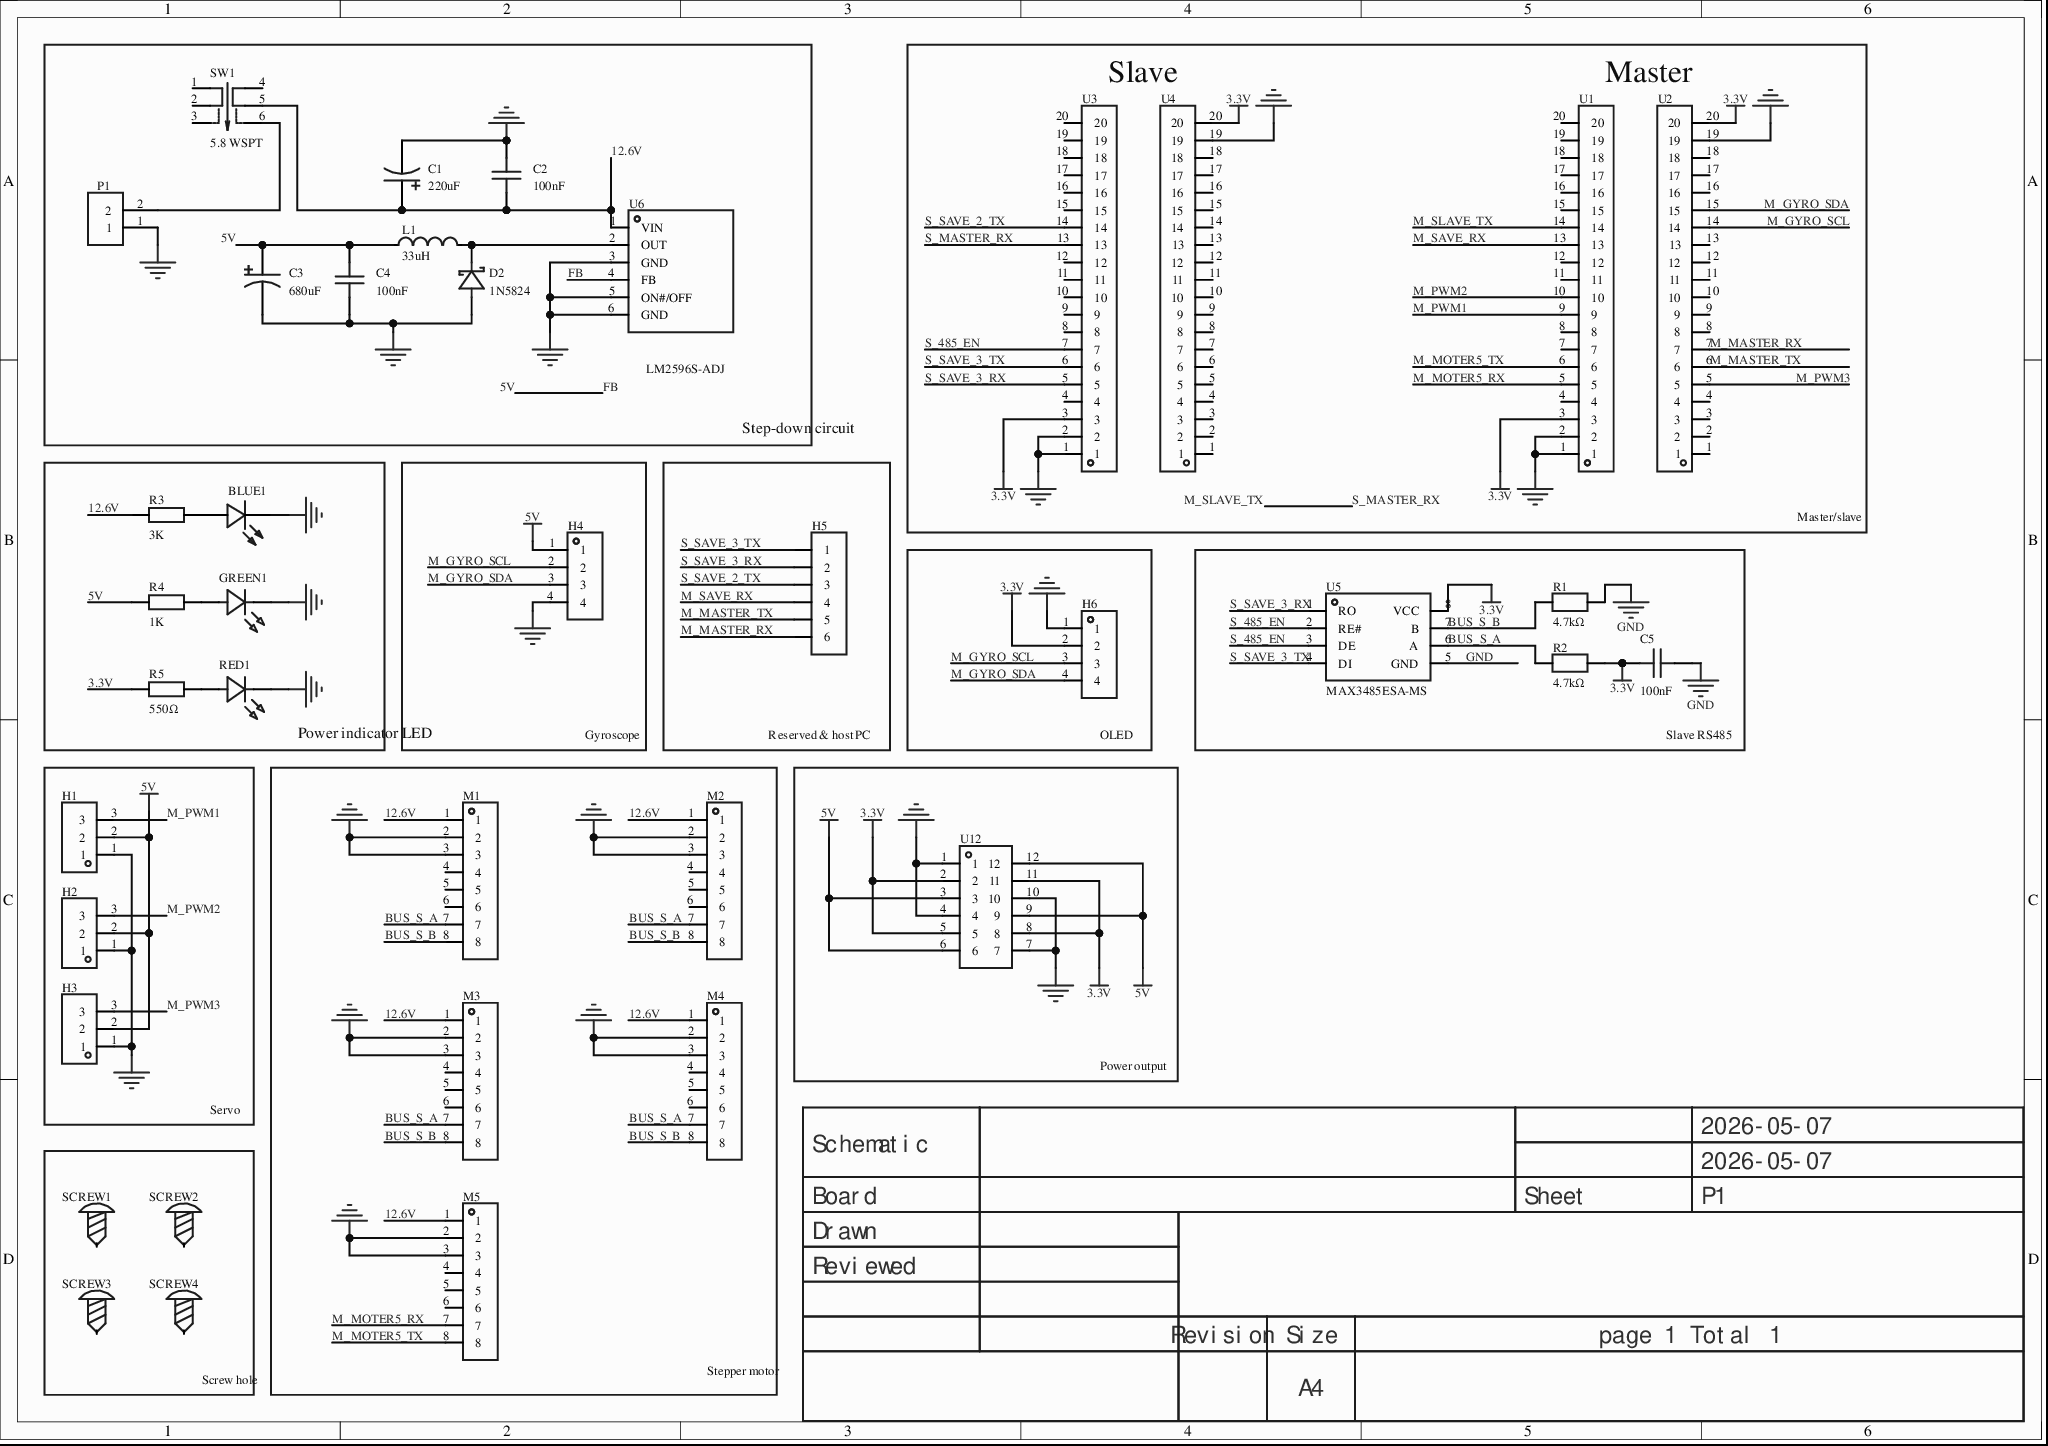
[diagram p0: MISC50151-3.schdoc]
# Altium project MISC50151-2.PrjPcb
1 sheet, 39 parts. Net scope: global (net labels, ports and power ports of the same name join across sheets).
Board file: MISC50151.pcbdoc

## Sheet MISC50151-3.schdoc
size 297 x 209 mm; Version: V1.0; @Project Name: MISC50151; @Page Count: 1; @Update Date: 2026-05-07; @Create Date: 2026-05-07; @Schematic Name: MISC50151; @Page No: 1; @Create Time: 22:11:46; @Update Time: 23:26:42; @Board Name: MISC50151

### Parts
BLUE1  SZYY0603B  [LED0603-R-RD_BLUE]  (value not drawn)
C1  220uF  [CAP-SMD_BD10.0-L10.3-W10.3-FD]
C2  100nF  [C0805]
C3  680uF  [CAP-SMD_BD8.0-L8.3-W8.3-FD]
C4  100nF  [C0805]
C5  100nF  [C0603]
D2  1N5824  [DO-27_BD5.3-L8.4-P12.40-D1.3-RD]
GREEN1  XL-1608PGC-06  [LED0603-RD_GREEN]  (value not drawn)
H1  PZ254V-11-03P  [HDR-TH_3P-P2.54-V-M]  (value not drawn)
H2  PZ254V-11-03P  [HDR-TH_3P-P2.54-V-M]  (value not drawn)
H3  PZ254V-11-03P  [HDR-TH_3P-P2.54-V-M]  (value not drawn)
H4  PZ254V-11-04P  [HDR-TH_4P-P2.54-V-M]  (value not drawn)
H5  2.54-1x6P straight pin  [HDR-TH_6P-P2.54-V-M-1]  (value not drawn)
H6  PZ254V-11-04P  [HDR-TH_4P-P2.54-V-M]  (value not drawn)
L1  33uH  [IND-SMD_L13.45-W12.6]
M1  ZX-XH2.54-8PWZ  [CONN-TH_8P-P2.50_ZX-XH2.54-8PWZ]  (value not drawn)
M2  ZX-XH2.54-8PWZ  [CONN-TH_8P-P2.50_ZX-XH2.54-8PWZ]  (value not drawn)
M3  ZX-XH2.54-8PWZ  [CONN-TH_8P-P2.50_ZX-XH2.54-8PWZ]  (value not drawn)
M4  ZX-XH2.54-8PWZ  [CONN-TH_8P-P2.50_ZX-XH2.54-8PWZ]  (value not drawn)
M5  ZX-XH2.54-8PWZ  [CONN-TH_8P-P2.50_ZX-XH2.54-8PWZ]  (value not drawn)
P1  WJ500V-5.08-2P  [CONN-TH_2P-P5.00_WJ500V-5.08-2P]  (value not drawn)
R1  4.7kΩ  [R0805]
R2  4.7kΩ  [R0805]
R3  3K  [R0805]
R4  1K  [R0805]
R5  550Ω  [R0805]
RED1  XL-1608SURC-06  [LED0603-RD_RED]  (value not drawn)
SCREW1  (no value)  [M3螺丝]
SCREW2  (no value)  [M3螺丝]
SCREW3  (no value)  [M3螺丝]
SCREW4  (no value)  [M3螺丝]
SW1  5.8 WSPT  [SW-TH_6P-L5.8-W5.8-P2.00-LS4.5-TL_K8-5851E-L1]
U1  ZX-PM2.54-1-20PY  [HDR-TH_20P-P2.54-V-F]  (value not drawn)
U2  ZX-PM2.54-1-20PY  [HDR-TH_20P-P2.54-V-F]  (value not drawn)
U3  ZX-PM2.54-1-20PY  [HDR-TH_20P-P2.54-V-F]  (value not drawn)
U4  ZX-PM2.54-1-20PY  [HDR-TH_20P-P2.54-V-F]  (value not drawn)
U5  MAX3485ESA-MS  [SO-8_L4.9-W3.9-P1.27-LS5.9-BL]
U6  LM2596S-ADJ  [TO-263-5_L10.2-W8.6-P1.70-LS14.4-BR]
U12  HX PZ2.54-3x4P ZZ  [HDR-TH_12P-P2.54-V-M-R3-C4-S2.54]  (value not drawn)

### Blocks framed on the sheet
Step-down circuit: C1-C4 D2 L1 P1 SW1 U6
Power indicator LED: BLUE1 GREEN1 R3-R5 RED1
Gyroscope: H4
Reserved & host PC: H5
OLED: H6
Slave RS485: C5 R1 R2 U5
Servo: H1-H3
Stepper motor: M1-M5
Power output: U12
Screw hole: SCREW1-SCREW4

### Nets
3.3V: C5.1 H6.2 R2.2 R5.2 U1.3 U2.20 U3.3 U4.20 U5.8(VCC) U12.2 U12.5 U12.8 U12.11
5V: C3.1 C4.2 H1.2 H2.2 H3.2 H4.1 L1.1 R4.2 U6.4(FB) U12.3 U12.6 U12.9 U12.12  [also labelled FB]
GND: BLUE1.2(-) C1.2 C2.1 C3.2 C4.1 C5.2 D2.2(A) GREEN1.1(K) H1.1 H2.1 H3.1 H4.4 H6.1 M1.2 M1.3 M2.2 M2.3 M3.2 M3.3 M4.2 M4.3 M5.2 M5.3 P1.1 R1.2 RED1.1(K) U1.1 U1.2 U2.19 U3.1 U3.2 U4.19 U5.5(GND) U6.3(GND) U6.5(ON#/OFF) U6.6(GND) U12.1 U12.4 U12.7 U12.10
12.6V: C1.1 C2.2 M1.1 M2.1 M3.1 M4.1 M5.1 R3.2 SW1.5 U6.1(VIN)
BUS_S_A: M1.7 M2.7 M3.7 M4.7 R2.1 U5.6(A)
BUS_S_B: M1.8 M2.8 M3.8 M4.8 R1.1 U5.7(B)
M_GYRO_SCL: H4.2 H6.3 U2.14
M_GYRO_SDA: H4.3 H6.4 U2.15
M_MASTER_RX: H5.6 U2.7
M_MASTER_TX: H5.5 U2.6
M_MOTER5_RX: M5.7 U1.5
M_MOTER5_TX: M5.8 U1.6
M_PWM1: H1.3 U1.9
M_PWM2: H2.3 U1.10
M_PWM3: H3.3 U2.5
M_SAVE_RX: H5.4 U1.13
M_SLAVE_TX: U1.14 U3.13  [also labelled S_MASTER_RX]
S_485_EN: U3.7 U5.2(RE#) U5.3(DE)
S_SAVE_2_TX: H5.3 U3.14
S_SAVE_3_RX: H5.2 U3.5 U5.1(RO)
S_SAVE_3_TX: H5.1 U3.6 U5.4(DI)
NetBLUE1_1: BLUE1.1(+) R3.1
NetD2_1: D2.1(K) L1.2 U6.2(OUT)
NetGREEN1_2: GREEN1.2(A) R4.1
NetP1_2: P1.2 SW1.6
NetR5_1: R5.1 RED1.2(A)

Not connected (* = marked no-connect by the designer): M1 4* 5* 6*; M2 4* 5* 6*; M3 4* 5* 6*; M4 4* 5* 6*; M5 4* 5* 6*; SCREW1 1*; SCREW2 1*; SCREW3 1*; SCREW4 1*; SW1 1* 2* 3* 4*; U1 4* 7* 8* 11* 12* 15* 16* 17* 18* 19* 20*; U2 1* 2* 3* 4* 8* 9* 10* 11* 12* 13* 16* 17* 18*; U3 4* 8* 9* 10* 11* 12* 15* 16* 17* 18* 19* 20*; U4 1* 2* 3* 4* 5* 6* 7* 8* 9* 10* 11* 12* 13* 14* 15* 16* 17* 18*

### Notes on the sheet
- Slave
- Master
- Master/slave
- 2026-05-07
- Schematic
- Board
- Sheet
- P1
- Drawn
- Reviewed
- Revision
- Size
- A4
- page 1 Total 1

### Library data of the parts
BLUE1 = SZYY0603B: Emitted color: Blue; Power: 100mW; Forward current: 5mA; Dominant wavelength: 460nm~475nm; Diode configuration: -; Lens color: Colorless transparent lens; Color temperature: -; Viewing angle: 120°; Packaging: -; Operating temperature: -40℃~+85℃;; Manufacturer: yongyu(永裕光电); AddInBom: yes; ModelId: 084ad08e1cd342ca871cc791b88f1a3a; ModelTransform: 63.7794,31.496,0,0,0,0,0,0,0; Peak Wavelength: 469nm; Symbol: SZYY0603B; Device: SZYY0603B; LCSC Part Name: 蓝灯; SupplierPart: C434421; ManufacturerPart: SZYY0603B; Supplier Footprint: 0603; JLCPCB Part Class: Extended library; Datasheet: https://example.com/upload/public/pdf/source/20191204/C434421_A4F05E4DF64B0F36639806529E783B5C.pdf; Supplier: LCSC; ConvertToPcb: yes; FootprintName: LED0603-R-RD_BLUE; ModelName: LED0603-R-RD_BLUE; Emitted Color: Blue; Power Dissipation: 100mW; Forward Current: 5mA; Dominant Wavelength: 460nm~475nm; Diode Configuration: -; Lens Color: Colorless transparent lens; Color Temperature: -; Viewing Angle: 120°; Mounting Sytle: -; Operating Temperature: -40℃~+85℃
C1 = EEEFK1H221P: Capacitance: 220uF; Tolerance: ±20%; Rated voltage: 50V; Capacitor body diameter: 10mm; Capacitor body length: 10.2mm; Ripple current: -; Equivalent series resistance: -; Operating life: 2000hrs@105℃; Operating temperature: -45℃~+105℃;; Manufacturer: PANASONIC(松下); AddInBom: yes; ModelId: b23815befd5e4172abc55cc8ac2654de; ModelTransform: 456.692,405.511,0,180,0,0,0,0,0; Device: EEEFK1H221P; Symbol: EEEFK1H221P; LCSC Part Name: 220uF±20%50V; SupplierPart: C178549; ManufacturerPart: EEEFK1H221P; Supplier Footprint: SMD,10x10.2mm; JLCPCB Part Class: ExtendedPart; Datasheet: https://example.com/upload/public/pdf/source/20180329/C178549_6E0EC09DB3BC10F05F8D4E4FCB841907.pdf; Supplier: LCSC; ConvertToPcb: yes; FootprintName: CAP-SMD_BD10.0-L10.3-W10.3-FD; ModelName: CAP-SMD_BD10.0-L10.3-W10.3-FD; Value: 220uF; Rated Voltage: 50V; φD: 10mm; L: 10.2mm; Ripple Current: -; Equivalent Series Resistance(ESR): -; Lifetime @ Temp: 2000hrs@105℃; Operating Temperature: -45℃~+105℃
C2 C4 = CAP_0805: ConvertToPcb: yes; SymbolName: CapAcitance; ModelId: 1ba041120af144c991958decab20d241; ModelName: C0805_L2.0-W1.3-H1.3; ModelTransform: 78.74,51.181,0,0,0,0,0,0.0005,0; Device: CAP_0805; AddInBom: yes; Supplier Footprint: 0805; FootprintName: C0805; Value: 100nF
C3 = EEEFP1V221AP: Capacitance: 220uF; Tolerance: ±20%; Rated voltage: 35V; Capacitor body diameter: 8mm; Capacitor body length: 10.2mm; Ripple current: -; Equivalent series resistance: -; Operating life: 2000hrs@105℃; Operating temperature: -45℃~+105℃;; Manufacturer: PANASONIC(松下); AddInBom: yes; ModelId: 5c9301d64f8b45ea89e061ac72e6cbf7; ModelTransform: 393.7,326.771,0,180,0,0,0,0,0; Value: 680uF; Device: EEEFP1V221AP; Symbol: EEEFP1V221AP; LCSC Part Name: 220uF ±20% 35V; ManufacturerPart: EEEFP1V221AP; Supplier Footprint: SMD,8x10.2mm; JLCPCB Part Class: Extended Part; Datasheet: https://example.com/upload/public/pdf/source/20181130/C278406_CB9CD87BC4579E70B6A89BF3334E5E7E.pdf; Supplier: LCSC; ConvertToPcb: yes; FootprintName: CAP-SMD_BD8.0-L8.3-W8.3-FD; ModelName: CAP-SMD_BD8.0-L8.3-W8.3-FD; Rated Voltage: 35V; φD: 8mm; L: 10.2mm; Ripple Current: -; Equivalent Series Resistance(ESR): -; Lifetime @ Temp: 2000hrs@105℃; Operating Temperature: -45℃~+105℃
C5 = CGA0603X7R104K500JT: Capacitance: 100nF; Tolerance: ±10%; Rated voltage: 50V; Temperature coefficient: X7R;; Manufacturer: HRE(芯声); AddInBom: yes; ModelId: ac125912035d415993ca9572d50418b10819f05c4eef4c71ace90d822a990e87; ModelName: C0603_L1.6-W0.8-H0.8; ModelTransform: 62.992,31.496,0,0,0,0,0,0,0; Symbol: CGA0603X7R104K500JT; Device: CGA0603X7R104K500JT; LCSC Part Name: 100nF ±10% 50V; SupplierPart: C6119867; ManufacturerPart: CGA0603X7R104K500JT; Supplier Footprint: 0603; JLCPCB Part Class: Extended Part; Datasheet: https://example.com/datasheet/CGA0603X7R104K500JT/7062573.html; Supplier: LCSC; ConvertToPcb: yes; FootprintName: C0603; Value: 100nF; Voltage Rating: 50V; Temperature Coefficient: X7R
D2 = 1N5824_C7503125: Diode configuration: Single; Forward voltage drop (Vf): 550mV@5A; DC reverse voltage (Vr): 30V; Rectified current: 5A;; Manufacturer: FUXINSEMI(富芯森美); AddInBom: yes; ModelId: 34c822afc58c4389bef282cc7fc2257f; ModelTransform: 578.739,207.771,0,0,0,0,0,0,-196.85; Reverse Leakage Current (Ir): 500uA@30V; Operating Junction Temperature Range: -55℃~+150℃; Non-Repetitive Peak Forward Surge Current: 150A; Symbol: 1N5824_C7503125; Device: 1N5824_C7503125; LCSC Part Name: 电压:30V 电流:5A; SupplierPart: C7503125; ManufacturerPart: 1N5824; Supplier Footprint: DO-201AD; JLCPCB Part Class: Extended library; Datasheet: https://example.com/datasheet/1N5824/8591231.html; Supplier: LCSC; ConvertToPcb: yes; FootprintName: DO-27_BD5.3-L8.4-P12.40-D1.3-RD; ModelName: DO-27_BD5.3-L8.4-P12.40-D1.3-RD; Diode Configuration: Single; Voltage - Forward(Vf@If): 550mV@5A; Voltage - DC Reverse(Vr): 30V; Current - Rectified: 5A
GREEN1 = XL-1608PGC-06: Lamp head type: -; Emitted color: Emerald green; Forward voltage (Vf): 2.6V~3V; Power: -; Forward current: -; Wavelength: 515nm~530nm; Diode configuration: -; Lens color: Green lens; Color temperature: -; Luminous intensity: 900mcd; Viewing angle: 120°; Packaging: SMD; Operating temperature: -;; Manufacturer: XINGLIGHT(成兴光); AddInBom: yes; ModelId: 7761174b67d9475ab0dbce38062fb2f9; ModelTransform: 63.7794,31.496,0,0,0,0,0,0,0; Peak Wavelength: 525nm; Symbol: XL-1608PGC-06; Device: XL-1608PGC-06; LCSC Part Name: 0603加粉翠绿0.6T贴片式发光二极管; SupplierPart: C7371905; ManufacturerPart: XL-1608PGC-06; Supplier Footprint: 0603; JLCPCB Part Class: Extended library; Datasheet: https://example.com/datasheet/XL-1608PGC-06/8342977.html; Supplier: LCSC; ConvertToPcb: yes; FootprintName: LED0603-RD_GREEN; ModelName: LED0603-RD_GREEN; Lamp Holder Type: -; Illumination Color: Emerald green; Voltage - Forward(Vf): 2.6V~3V; Power(Watts): -; Forward Current: -; Wavelength - Dominant: 515nm~530nm; Diode Configuration: -; Lens Color: Green lens; Color Temperature: -; Luminous Intensity: 900mcd; Viewing Angle: 120°; Mounting Style: SMD; Operating Temperature: -
H1-H3 = PZ254V-11-03P: Pin structure: 1x3P; Pitch: 2.54mm; Row spacing: -; Round/square pin: Square pin; Mounting style: Through-hole; Rows: Single row; Total pins: 3P; Rated current: 3A; Rated voltage: 250V; Mating pin length: 6mm; Plastic height: 2.5mm; Tail length: 3mm; Operating temperature: -40℃~+105℃; Color: Black;; Manufacturer: XFCN(兴飞); Symbol: PZ254V-11-03P_C2937625; AddInBom: yes; ModelId: bb473b6d38ff42a99216a4fcdbdcc4cb; ModelName: HDR-TH_3P-P2.54-M-LI-1X3P; ModelTransform: 299.9994,100,0,0,0,0,0,0,-118.11; Device: PZ254V-11-03P; LCSC Part Name: 1x3P 间距:2.54mm 方针 直插; SupplierPart: C2937625; ManufacturerPart: PZ254V-11-03P; Supplier Footprint: 插件,P=2.54mm; JLCPCB Part Class: Extended library; Datasheet: https://example.com/datasheet/PZ254V-11-03P/3293280.html; Supplier: LCSC; ConvertToPcb: yes; FootprintName: HDR-TH_3P-P2.54-V-M; Pin Structure: 1x3P; Row Spacing: -; Circluar Pins/Square Pins: Square pin; Mounting Type: Through-hole; Number of Rows: Single row; Number of Pins: 3P; Current Rating: 3A; Voltage Rating (Max): 250V; Length of Mating Pin: 6mm; Insulation Height: 2.5mm; Length of End Connection Pin: 3mm; Operating Temperature: -40℃~+105℃; Color: Black
H4 H6 = PZ254V-11-04P: Pin structure: 1x4P; Pitch: 2.54mm; Row spacing: -; Round/square pin: Square pin; Mounting style: Through-hole; Rows: Single row; Total pins: 4P; Rated current: 3A; Rated voltage: 250V; Mating pin length: 6mm; Plastic height: 2.5mm; Tail length: 3mm; Contact material: -; Operating temperature: -40℃~+105℃;; Manufacturer: XFCN(兴飞); Symbol: PZ254V-11-04P_C2691448; AddInBom: yes; ModelId: 112f4d05e8d64e99ab9a333894bea4f9; ModelName: HDR-TH_4P-P2.54-M-LI-1X4P; ModelTransform: 399.999,104.7242,0,0,0,0,0,0,-118.11; Device: PZ254V-11-04P; LCSC Part Name: 1x4P 间距:2.54mm 方针 直插; SupplierPart: C2691448; ManufacturerPart: PZ254V-11-04P; Supplier Footprint: 插件,P=2.54mm; JLCPCB Part Class: Extended library; Datasheet: https://example.com/datasheet/PZ254V-11-04P/2801085.html; Supplier: LCSC; ConvertToPcb: yes; FootprintName: HDR-TH_4P-P2.54-V-M; Pin Structure: 1x4P; Row Spacing: -; Circluar Pins/Square Pins: Square pin; Mounting Type: Through-hole; Number of Rows: Single row; Number of Pins: 4P; Current Rating: 3A; Voltage Rating (Max): 250V; Length of Mating Pin: 6mm; Insulation Height: 2.5mm; Length of End Connection Pin: 3mm; Contact Material: -; Operating Temperature: -40℃~+105℃; Color: Black
H5 = 2.54-1x6P直针: Pin structure: 1x6P; Pitch: 2.54mm; Row spacing: -; Round/square pin: Square pin; Mounting style: Through-hole; Rows: Single row; Total pins: 6P; Rated current: 3A; Rated voltage: -; Mating pin length: 6mm; Plastic height: 2.5mm; Tail length: 3mm; Contact material: Brass; Contact plating: Gold; Operating temperature: -40℃~+105℃; Color: Black;; Manufacturer: BOOMELE(博穆精密); Symbol: Header-Male-2.54_1x6; AddInBom: yes; ModelId: 60739dffc9b04830a286435b0fefbd4a; ModelName: HDR2.54-M-LI-1X6P; ModelTransform: 599.999,100,0,0,0,0,0,0,-118.11; Device: 2.54-1x6P straight pin; LCSC Part Name: 1x6P 间距:2.54mm 方针 直插; SupplierPart: C37208; ManufacturerPart: 2.54-1x6P直针; Supplier Footprint: 插件,P=2.54mm; JLCPCB Part Class: Extended library; Datasheet: https://example.com/datasheet/2.54-1x6P%25E7%259B%25B4%25E9%2592%2588/38187.html; Supplier: LCSC; ConvertToPcb: yes; FootprintName: HDR-TH_6P-P2.54-V-M-1; Pin Structure: 1x6P; Row Spacing: -; Circluar Pins/Square Pins: Square pin; Mounting Type: Through-hole; Number of Rows: Single row; Number of Pins: 6P; Current Rating: 3A; Voltage Rating (Max): -; Length of Mating Pin: 6mm; Insulation Height: 2.5mm; Length of End Connection Pin: 3mm; Contact Material: Brass; Contact Plating: Gold; Operating Temperature: -40℃~+105℃; Color: Black
L1 = MWSA1206S-330MT: Type: -; Inductance: 33uH; Tolerance: ±20%; Rated current: 5.5A; Saturation current (Isat): 6A;; Manufacturer: Sunlord(顺络); AddInBom: yes; ModelId: 5e32e44c45c84c74ac625f8e46b1bee3; ModelName: IND-SMD_L13.45-W12.6-H4.8; ModelTransform: 529.5265,496.062,0,0,0,0,0,0,0; DC Resistance (DCR): 75mΩ; Device: MWSA1206S-330MT; Symbol: MWSA1206S-330MT; LCSC Part Name: 33uH±20%6A; SupplierPart: C408530; ManufacturerPart: MWSA1206S-330MT; Supplier Footprint: SMD; JLCPCB Part Class: ExtendedPart; Datasheet: https://example.com/upload/public/pdf/source/20191101/C408530_8564194D40E02E1E74EF0675498FAD8D.pdf; Supplier: LCSC; ConvertToPcb: yes; FootprintName: IND-SMD_L13.45-W12.6; Value: 33uH; Rated Current: 5.5A; Saturation Current (Isat): 6A; Ratings: -
M1-M5 = ZX-XH2.54-8PWZ: Pin structure: 1x8P; Pitch: 2.5mm; Mounting style: Right angle; Reference series: XH; Total pins: 8P; Rows: 1; Pins per row: 8; Row spacing: -; Rated current: 3A; Contact material: Brass; Contact plating: Tin; Operating temperature: -25℃~+85℃;; Manufacturer: Megastar(兆星); AddInBom: yes; ModelId: 2313deb9a1954eec88de97710f9a8a07; ModelTransform: 886.2187,300.7868,0,0,0,0,-0.002,-137.795,-133.858; Number of PINs Per Row: 8; Voltage Rating: 250V; Plastic Material: PA66; Flame Retardant Rating: UL94V-0; Z-Height of the Board: 5.9mm; X-Length of Bottom Edge on Board (Spacing Line): 22.5mm; Y-Width of Bottom Edge on Board: 7.32mm; Symbol: ZX-XH2.54-8PWZ; Device: ZX-XH2.54-8PWZ; LCSC Part Name: 1x8P 间距:2.5mm 弯插 系列:XH; SupplierPart: C7429647; ManufacturerPart: ZX-XH2.54-8PWZ; Supplier Footprint: 弯插,P=2.5mm; JLCPCB Part Class: Extended library; Datasheet: https://example.com/datasheet/ZX-XH2.54-8PWZ/8427564.html; Supplier: LCSC; ConvertToPcb: yes; FootprintName: CONN-TH_8P-P2.50_ZX-XH2.54-8PWZ; ModelName: CONN-TH_8P-P2.50_ZX-XH2.54-8PWZ; Pins Structure: 1x8P; Mounting Type: Right angle; Reference Series: XH; Number of Pins: 8P; Number of Rows: 1; Row Spacing: -; Current Rating: 3A; Contact Material: Brass; Contact Plating: Tin; Operating Temperature: -25℃~+85℃; Supplementary Features: -; Color: White
P1 = WJ500V-5.08-2P: Structure: 1x2P; Pitch: 5.08mm; Color: Green; Mounting style: Through-hole; Rated current: 18A; Rated voltage: 250V; Rows: 1; Wire gauge - AWG: 14~30; Wire gauge - mm²: 2.5; Pins per row: 2; Contact material: -; Contact plating: -; Operating temperature range: -40℃~+105℃; Soldering temperature (max): -;; Manufacturer: KANGNEX(康奈克斯电气); Symbol: WJ500V-5.08-2P-14-00A; AddInBom: yes; ModelId: 0f4a503c8d3b4ae19ed61267f5e9a1d7; ModelTransform: 423.621,393.7,0,0,0,0,-11.811,19.685,-137.795; Wire Gauge - mm2: 2.5; Number of PINs Per Row: 2; Screw Specification: M2.5; Device: WJ500V-5.08-2P; LCSC Part Name: 1x2P 5.08mm 直插 排数:1 每排P数:2; SupplierPart: C8465; ManufacturerPart: WJ500V-5.08-2P; Supplier Footprint: 插件,P=5.08mm; JLCPCB Part Class: Extended library; Datasheet: https://example.com/upload/public/pdf/source/20191225/C8465_02D34CE5B5B4A53DF5891601D97FA9F4.pdf; Supplier: LCSC; ConvertToPcb: yes; FootprintName: CONN-TH_2P-P5.00_WJ500V-5.08-2P; ModelName: CONN-TH_2P-P5.00_WJ500V-5.08-2P; Mounting Style: Through-hole; Current Rating (Max): 18A; Voltage Rating (Max): 250V; Number of Pins: 2P; Number of Rows: 1; Wire Gauge - AWG: 14~30; Contact Material: -; Contact Plating: -; Operating Temperature Range: -40℃~+105℃; Soldering Temperature(Max): -
R1 R2 = FRC0402F1002TS: Resistor type: Thick film resistor; Resistance: 10kΩ; Tolerance: ±1%; Power: 62.5mW; Operating voltage: 50V; Temperature coefficient: ±100ppm/℃;; Manufacturer: FOJAN(富捷); AddInBom: yes; ModelId: 98c88bc2b9094f218f3a3e30a70127380819f05c4eef4c71ace90d822a990e87; ModelName: R0402_L1.0-W0.5-H0.4; ModelTransform: 39.37,19.685,0,0,0,0,0,0,0; Symbol: FRC0402F1002TS; Device: FRC0402F1002TS; Value: 4.7kΩ; LCSC Part Name: 10kΩ ±1% 62.5mW 厚膜电阻; ManufacturerPart: FRC0402F1002TS; Supplier Footprint: 0402; JLCPCB Part Class: Extended Part; Datasheet: https://example.com/datasheet/FRC0402F1002TS/3180374.html; Supplier: LCSC; ConvertToPcb: yes; FootprintName: R0805; Type: Thick film resistor; Power(Watts): 62.5mW; Voltage-Supply(Max): 50V; Temperature Coefficient: ±100ppm/℃; Operating Temperature: -55℃~+155℃
R3-R5 = Res_0805: Symbol: Resistor; ConvertToPcb: yes; ModelId: 37a81e68749a4138bd2dfa6897b24b85; ModelName: R0805_L2.0-W1.3-H0.6; ModelTransform: 78.74,51.181,0,0,0,0,0,-0.0005,0; Device: Res_0805; AddInBom: yes; Supplier Footprint: 0805; FootprintName: R0805
  R3: Value: 3K
  R4: Value: 1K
  R5: Value: 550Ω
RED1 = XL-1608SURC-06: Lamp head type: -; Emitted color: Red; Forward voltage (Vf): 2.3V; Power: 50mW; Forward current: 20mA; Wavelength: 620nm~630nm; Diode configuration: -; Lens color: Colorless transparent lens; Color temperature: -; Luminous intensity: 225mcd; Viewing angle: 120°; Packaging: SMD; Operating temperature: -40℃~+85℃;; Manufacturer: XINGLIGHT(成兴光); AddInBom: yes; ModelId: 74041d3a270d435c8600a9ab9b7641c0; ModelTransform: 63.7794,31.496,0,0,0,0,0,0,0; Peak Wavelength: 625nm; Symbol: XL-1608SURC-06; Device: XL-1608SURC-06; LCSC Part Name: 0603红色贴片式发光二极管; SupplierPart: C965799; ManufacturerPart: XL-1608SURC-06; Supplier Footprint: 0603; JLCPCB Part Class: Extended library; Datasheet: https://example.com/datasheet/XL-1608SURC-06/1051408.html; Supplier: LCSC; ConvertToPcb: yes; FootprintName: LED0603-RD_RED; ModelName: LED0603-RD_RED; Lamp Holder Type: -; Illumination Color: Red; Voltage - Forward(Vf): 2.3V; Power(Watts): 50mW; Forward Current: 20mA; Wavelength - Dominant: 620nm~630nm; Diode Configuration: -; Lens Color: Colorless transparent lens; Color Temperature: -; Luminous Intensity: 225mcd; Viewing Angle: 120°; Mounting Style: SMD; Operating Temperature: -40℃~+85℃
SCREW1-SCREW4 = M3螺丝: Device: M3 screw; ConvertToPcb: yes; SymbolName: Screw hole; AddInBom: yes; Supplier Footprint: 插件; FootprintName: M3 screw
SW1 = 5.8 WSPT: Circuit structure: DPDT; Self-lock/no-lock: No lock; Mounting style: Through-hole; Contact current: 100mA; Rated voltage: 30V; Lamp: No; Actuating force: 1.8N; Operating life: 5 thousand cycles;; Manufacturer: SHOU HAN(首韩); 3D Model: b8faad98a5c645e9866333cdaba903c3; 3D Model Transform: 229.1334,228.346,0,0,0,0,0,0,-137.795; Self Lock / No Lock: No lock; Actuator Style: Rectangular plunger; Actuator/Cap Color: Blue; AddInBom: yes; Symbol: 5.8 WSPT; Device: 5.8 WSPT; LCSC Part Name: 按键开关5.8x5.8 无锁平头 180gf; Supplier Part: C5379898; Manufacturer Part: 5.8 WSPT; Supplier Footprint: 插件; JLCPCB Part Class: Extended library; Datasheet: https://example.com/datasheet/5.8%2520WSPT/6245006.html; Supplier: LCSC; Circuit: DPDT; IP Rating: -; Mounting Type: Through-hole; Contact Current: 100mA; Voltage Rating: 30V; With Lamp: No; Termination Style: PC pin; Operating Force: 1.8N; Operating Temperature: -10℃~+70℃; Life: 5 thousand cycles; ConvertToPcb: yes; FootprintName: SW-TH_6P-L5.8-W5.8-P2.00-LS4.5-TL_K8-5851E-L1; ModelName: SW-TH_6P-L5.8-W5.8-P2.00-LS4.5-TL_K8-5851E-L1
U1-U4 = ZX-PM2.54-1-20PY: Socket structure: 1x20P; Pitch: 2.54mm; Row spacing: -; Round/square hole: Square hole; Mounting type: Through-hole; Rows: Single row; Total holes: 20P; Rated current: -; Rated voltage: 1kV; Socket direction: Top; Plastic height: 8.5mm; Contact material: -; Contact plating: Gold; Operating temperature range: -40℃~+105℃;; Manufacturer: Megastar(兆星); AddInBom: yes; ModelId: db7015f7ad9d48b8a3b1188db02e3429; ModelName: HDR-F-2.54_1x20; ModelTransform: 1999.996,100,0,0,0,0,0,0,-118.11; Symbol: ZX-PM2.54-1-20PY; Device: ZX-PM2.54-1-20PY; LCSC Part Name: 1x20P 间距:2.54mm 直插; SupplierPart: C7499336; ManufacturerPart: ZX-PM2.54-1-20PY; Supplier Footprint: 插件,P=2.54mm; JLCPCB Part Class: Extended library; Datasheet: https://example.com/upload/public/pdf/source/20231122/D07E8E83FD020EE141D56DDF9758AF41.pdf; Supplier: LCSC; ConvertToPcb: yes; FootprintName: HDR-TH_20P-P2.54-V-F; Holes Structure: 1x20P; Row Spacing: -; Circular Hole / Square Hole: Square hole; Mounting Type: Through-hole; Number of Rows: Single row; Number of Holes: 20P; Current Rating (Max): -; Voltage Rating (Max): 1kV; Holes Direction: Top; Insulation Height: 8.5mm; Contact Material: -; Contact Plating: Gold; Operating Temperature Range: -40℃~+105℃
U5 = MAX3485ESA-MS: Type: Transceiver; Data rate: 12Mbps;; Manufacturer: MSKSEMI(美森科); AddInBom: yes; ModelId: 756fba4e187a48c69a2c935cd5c4465b0819f05c4eef4c71ace90d822a990e87; ModelName: SO-8_L4.9-W3.9-H1.5-LS5.9-P1.27; ModelTransform: 240.39054,192.913,0,270,0,0,0.0005,-0.0005,0; Number of Drivers: 1; Voltage - Supply: 3V~5.5V; Number of Nodes: 256; ESD Protect: ±15kV; Communication Mode: Half-duplex; Symbol: MAX3485ESA-MS; Device: MAX3485ESA-MS; LCSC Part Name: MAX3485E RS-485 收发器; SupplierPart: C7434431; ManufacturerPart: MAX3485ESA-MS; Supplier Footprint: SOP-8; JLCPCB Part Class: Extended Part; Datasheet: https://example.com/datasheet/MAX3485ESA-MS/8445950.html; Supplier: LCSC; ConvertToPcb: yes; FootprintName: SO-8_L4.9-W3.9-P1.27-LS5.9-BL; Number of Receivers: 1; Data Rate: 12Mbps; Operating Temperature: -40℃~+125℃
U6 = LM2596S-ADJ_C5276751: Manufacturer: TWGMC(台湾迪嘉); AddInBom: yes; ModelId: 95ee68e4aae845298b3c6638974e3d4a; ModelTransform: 399.999,564.96,0,90,0,0,-60.197,0,0; Device: LM2596S-ADJ_C5276751; Symbol: LM2596S-ADJ_C5276751; LCSC Part Name: LM2596S-ADJ; SupplierPart: C5276751; ManufacturerPart: LM2596S-ADJ; Supplier Footprint: TO-263-5; JLCPCB Part Class: ExtendedPart; Datasheet: https://example.com/upload/public/pdf/source/20221121/1586C0ED4283566B84D2D5018D7561E0.pdf; Supplier: LCSC; ConvertToPcb: yes; FootprintName: TO-263-5_L10.2-W8.6-P1.70-LS14.4-BR; ModelName: TO-263-5_L10.2-W8.6-P1.70-LS14.4-BR
U12 = HX PZ2.54-3x4P ZZ: Pin structure: 3x4P; Pitch: 2.54mm; Row spacing: 2.54mm; Round/square pin: Square pin; Mounting style: Through-hole; Rows: Three rows; Total pins: 12P; Rated current: 3A; Rated voltage: 1kV; Mating pin length: 6mm; Plastic height: 2.5mm; Tail length: 3mm; Contact material: Brass; Contact plating: Gold; Operating temperature: -40℃~+105℃; Color: Black;; Manufacturer: hanxia(韩下); AddInBom: yes; ModelId: a7ddfe346b9649f096e65c72c89ac56b; ModelTransform: 399.999,298.4246,0,0,0,0,0,0,-118.11; Symbol: HX PZ2.54-3X4P ZZ; Device: HX PZ2.54-3x4P ZZ; LCSC Part Name: 3x4P 间距:2.54mm 方针 直插; SupplierPart: C32713291; ManufacturerPart: HX PZ2.54-3x4P ZZ; Supplier Footprint: 插件,P=2.54mm; JLCPCB Part Class: Extended library; Datasheet: https://example.com/datasheet/HX%2520PZ2.54-3x4P%2520ZZ/34444571.html; Supplier: LCSC; ConvertToPcb: yes; FootprintName: HDR-TH_12P-P2.54-V-M-R3-C4-S2.54; ModelName: HDR-TH_12P-P2.54-V-M-R3-C4-S2.54; Pin Structure: 3x4P; Row Spacing: 2.54mm; Circluar Pins/Square Pins: Square pin; Mounting Type: Through-hole; Number of Rows: Three rows; Number of Pins: 12P; Current Rating: 3A; Voltage Rating (Max): 1kV; Length of Mating Pin: 6mm; Insulation Height: 2.5mm; Length of End Connection Pin: 3mm; Contact Material: Brass; Contact Plating: Gold; Operating Temperature: -40℃~+105℃; Color: Black; Supplementary Features: -